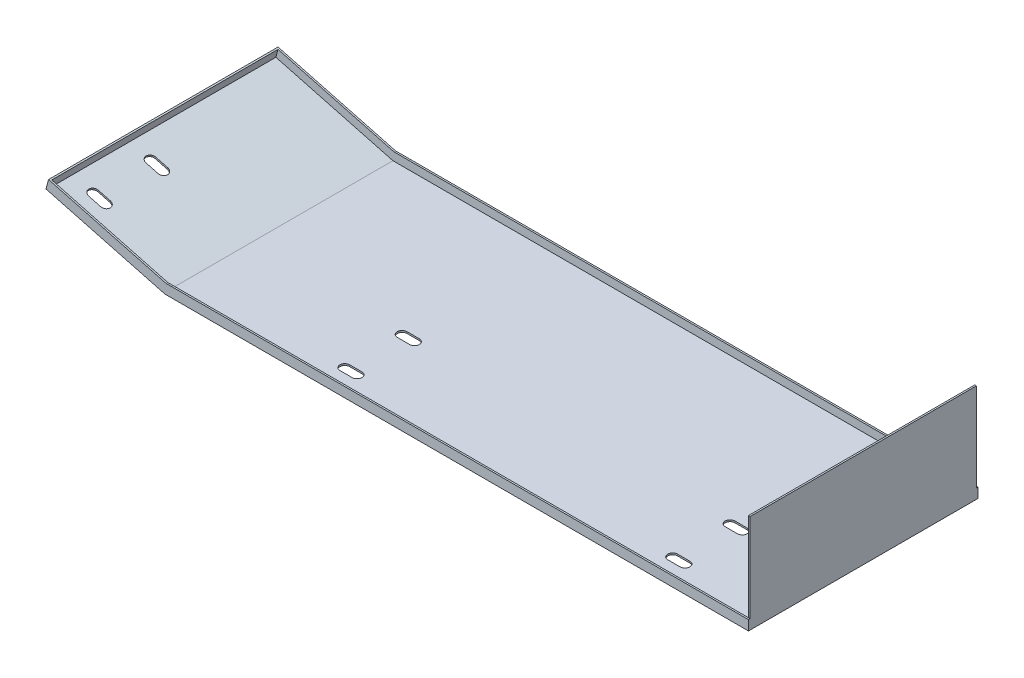
from build123d import *

# Parameters (mm, degrees)
EXTRUDE_THIN1_DEPTH  = 276
EXTRUDE_THIN2_DEPTH  = 2
EXTRUDE_THIN3_DEPTH  = 2
CUT_EXTRUDE1_DEPTH   = 2
LPATTERN1_COUNT      = 2
LPATTERN1_PITCH      = 400
LPATTERN1_COUNT_DIR2 = 2
LPATTERN1_PITCH_DIR2 = 70
CUT_EXTRUDE2_DEPTH   = 2
LPATTERN2_COUNT      = 2
LPATTERN2_PITCH      = 70
SKETCH7_W            = 2
SKETCH7_H            = 276
BOSS_EXTRUDE1_DEPTH  = 10


with BuildPart() as part:
    # Sketch1 → Extrude-Thin1 (new body)
    with BuildSketch(Plane.XY):
        Polygon((-856.990015303, 38.44340597), (-712, 0), (0, 0), (0, 120), (-2, 120), (-2, 2), (-711.739357917, 2), (-856.477436556, 40.376606174), align=None)
    extrude(amount=EXTRUDE_THIN1_DEPTH)

    # Sketch2 → Extrude-Thin2 (add)
    with BuildSketch(Plane.XY.offset(276)):
        Polygon((0, 0), (-712, 0), (-856.990015303, 38.44340597), (-853.914542825, 50.042607194), (-710.436147504, 12), (0, 12), align=None)
    extrude(amount=EXTRUDE_THIN2_DEPTH)

    # Sketch4 → Extrude-Thin3 (add)
    with BuildSketch(Plane(origin=(0, 0, 0), x_dir=(-1, 0, 0), z_dir=(0, 0, -1))):
        Polygon((0, 0), (712, 0), (856.990015303, 38.44340597), (853.914542825, 50.042607194), (710.436147504, 12), (0, 12), align=None)
    extrude(amount=EXTRUDE_THIN3_DEPTH)

    # Sketch5 → Cut-Extrude1 (cut)
    with BuildSketch(Plane.XZ):
        with BuildLine():
            Line((-122.5, 254), (-107.5, 254))
            ThreePointArc((-107.5, 254), (-101.5, 248), (-107.5, 242))
            Line((-107.5, 242), (-122.5, 242))
            ThreePointArc((-122.5, 242), (-128.5, 248), (-122.5, 254))
        make_face()
    cut_extrude1 = extrude(amount=-CUT_EXTRUDE1_DEPTH, mode=Mode.SUBTRACT)

    # LPattern1: Cut-Extrude1 2 × 2
    with Locations(*[(-i * LPATTERN1_PITCH, 0, -j * LPATTERN1_PITCH_DIR2) for i in range(LPATTERN1_COUNT) for j in range(LPATTERN1_COUNT_DIR2) if (i, j) != (0, 0)]):
        add(cut_extrude1, mode=Mode.SUBTRACT)

    # Sketch6 → Cut-Extrude2 (cut)
    with BuildSketch(Plane(origin=(-46.76718086, -176.383285962, 0), x_dir=(0.9666001020169073, -0.2562893731329973, 0), z_dir=(-0.2562893731329973, -0.9666001020169073, 0))):
        with BuildLine():
            Line((-809.719272636, 254), (-794.719272636, 254))
            ThreePointArc((-794.719272636, 254), (-788.719272636, 248), (-794.719272636, 242))
            Line((-794.719272636, 242), (-809.719272636, 242))
            ThreePointArc((-809.719272636, 242), (-815.719272636, 248), (-809.719272636, 254))
        make_face()
    cut_extrude2 = extrude(amount=-CUT_EXTRUDE2_DEPTH, mode=Mode.SUBTRACT)

    # LPattern2: Cut-Extrude2 ×2
    with Locations(*[(0, 0, -i * LPATTERN2_PITCH) for i in range(1, LPATTERN2_COUNT)]):
        add(cut_extrude2, mode=Mode.SUBTRACT)

    # Sketch7 → Boss-Extrude1 (add)
    with BuildSketch(Plane(origin=(-46.254602114, -174.450085758, 0), x_dir=(0.9666001020169073, -0.25628937313299727, 0), z_dir=(0.25628937313299727, 0.9666001020169073, 0))):
        with Locations((-837.219272636, -138)):
            Rectangle(SKETCH7_W, SKETCH7_H)
    extrude(amount=BOSS_EXTRUDE1_DEPTH)


solid = part.part
